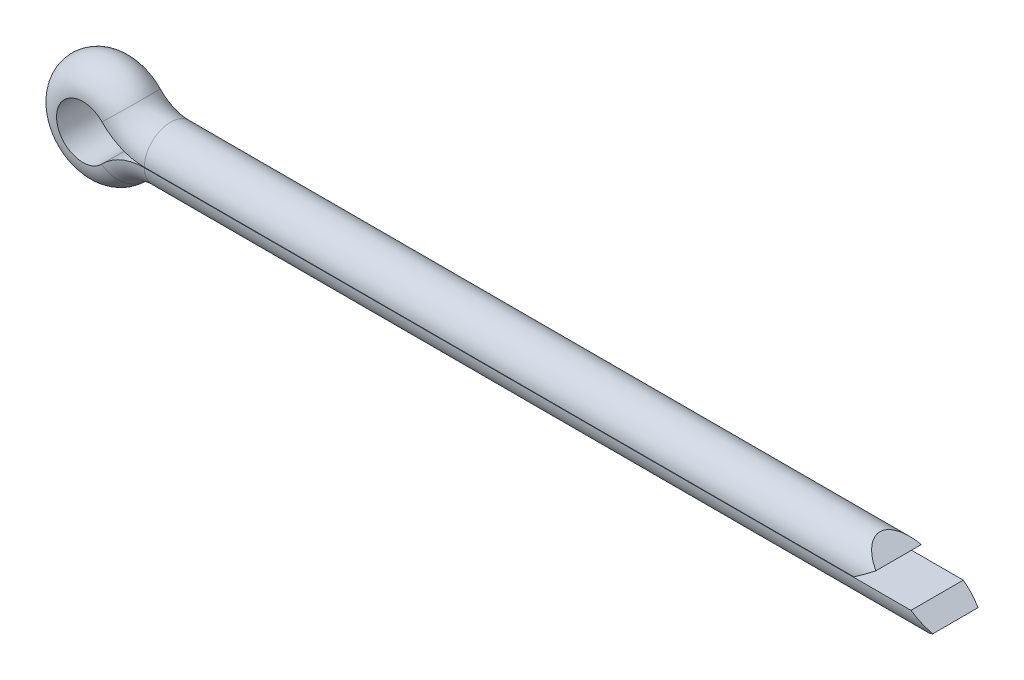
from build123d import *

# Parameters (mm, degrees)
CUT_EXTRUDE1_DEPTH      = 38.288770437
CUT_EXTRUDE1_DEPTH_BACK = 38.288770437


with BuildPart() as part:
    # Sweep2: sweep along a path in Dimension Sketch
    with BuildLine(Plane.XY) as sweep2_path:
        Line((34.7, 1.15), (2.7, 1.15))
        ThreePointArc((2.7, 1.15), (2.133929691, 1.265530578), (1.658403483, 1.593642961))
        ThreePointArc((1.658403483, 1.593642961), (-2.3, 0), (1.658403483, -1.593642961))
        ThreePointArc((1.658403483, -1.593642961), (2.133929691, -1.265530578), (2.7, -1.15))
        Line((2.7, -1.15), (37.2, -1.15))
    # Sketch2 → Sweep2 (sweep)
    with BuildSketch(Plane(origin=(34.7, 1.15, 0), x_dir=(0, 0, 1), z_dir=(-1, 0, 0))):
        with BuildLine():
            Line((-1.149956521, -1.14), (1.149956521, -1.14))
            ThreePointArc((1.149956521, -1.14), (0, 0), (-1.149956521, -1.14))
        make_face()
    sweep(path=sweep2_path.line)

    # Sketch3 → Cut-Extrude1 (cut, two sides: drawn at the far end of the back side and taken through both)
    with BuildSketch(Plane.XY.offset(-CUT_EXTRUDE1_DEPTH_BACK)):
        Polygon((34.7, 0.57), (33.882315934, 1.15), (37.21, 1.15), (37.21, -1.15), (36.375313858, -1.15), (37.2, -0.58), (36.382315934, 0), (33.875313858, 0), align=None)
    extrude(amount=CUT_EXTRUDE1_DEPTH + CUT_EXTRUDE1_DEPTH_BACK, mode=Mode.SUBTRACT)


solid = part.part
